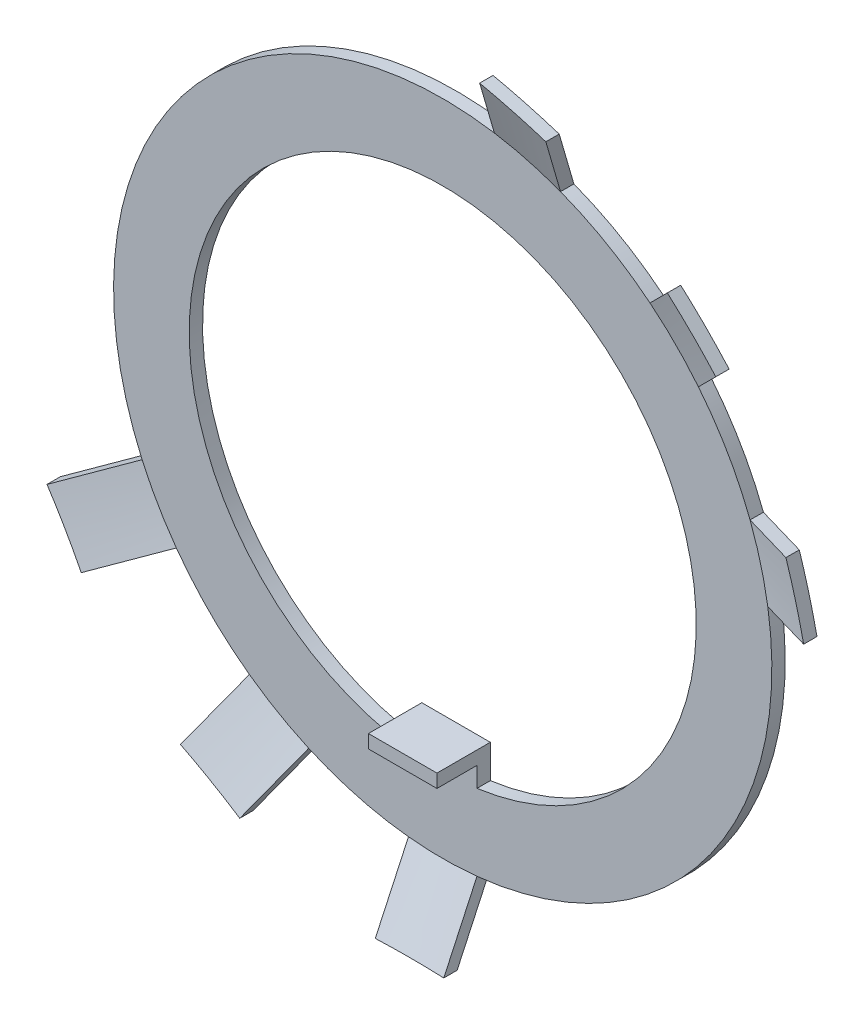
from build123d import *

# Parameters (mm, degrees)
SKETCH3_OUTSIDE_W   = 117.478
SKETCH3_OUTSIDE_H   = 117.478
CUT_EXTRUDE2_DEPTH  = 5.230463
SKETCH4_W           = 7.7
SKETCH4_H           = 1.5
BOSS_EXTRUDE1_DEPTH = 6


with BuildPart() as part:
    # Sketch2 → Boss-Revolve (revolve)
    with BuildSketch(Plane(origin=(0, 0, 0), x_dir=(0, 0, -1), z_dir=(1, 0, 0))):
        Polygon((-3.730461265, 45), (0, 37), (0, 0), (-1.5, 0), (-1.5, 37), (-5.230461265, 45), align=None)
    revolve(axis=Axis((0, 0, 0), (0, 0, 1)))

    # Sketch3 outside → Cut-Extrude2 (cut)
    # profile 1 of 2: a face of its own
    with BuildSketch(Plane.XY):
        Rectangle(SKETCH3_OUTSIDE_W, SKETCH3_OUTSIDE_H)
        with BuildLine():
            Line((-3.85, -36.799150805), (-3.85, -44.835003067))
            Line((-3.85, -44.835003067), (3.85, -44.835003067))
            Line((3.85, -44.835003067), (3.85, -36.799150805))
            ThreePointArc((3.85, -36.799150805), (29.354073591, -22.524172873), (36.541703472, 5.805506641))
            Line((36.541703472, 5.805506641), (44.303740708, 7.88533825))
            Line((44.303740708, 7.88533825), (42.31083406, 15.322967112))
            Line((42.31083406, 15.322967112), (34.548796825, 13.243135503))
            ThreePointArc((34.548796825, 13.243135503), (32.04293994, 18.5), (28.743290184, 23.298567969))
            Line((28.743290184, 23.298567969), (34.425495811, 28.980773595))
            Line((34.425495811, 28.980773595), (28.980773595, 34.425495811))
            Line((28.980773595, 34.425495811), (23.298567969, 28.743290184))
            ThreePointArc((23.298567969, 28.743290184), (18.5, 32.04293994), (13.243135503, 34.548796825))
            Line((13.243135503, 34.548796825), (15.322967112, 42.31083406))
            Line((15.322967112, 42.31083406), (7.88533825, 44.303740708))
            Line((7.88533825, 44.303740708), (5.805506641, 36.541703472))
            ThreePointArc((5.805506641, 36.541703472), (-29.354073591, 22.524172873), (-33.793999435, -15.065377598))
            Line((-33.793999435, -15.065377598), (-40.753251635, -19.083303729))
            Line((-40.753251635, -19.083303729), (-36.903251635, -25.751699338))
            Line((-36.903251635, -25.751699338), (-29.943999435, -21.733773207))
            ThreePointArc((-29.943999435, -21.733773207), (-26.162950904, -26.162950904), (-21.733773207, -29.943999435))
            Line((-21.733773207, -29.943999435), (-25.751699338, -36.903251635))
            Line((-25.751699338, -36.903251635), (-19.083303729, -40.753251635))
            Line((-19.083303729, -40.753251635), (-15.065377598, -33.793999435))
            ThreePointArc((-15.065377598, -33.793999435), (-9.576304669, -35.739255573), (-3.85, -36.799150805))
        make_face(mode=Mode.SUBTRACT)
    # profile 2 of 2: a face of its own
    with BuildSketch(Plane.XY):
        with BuildLine():
            Line((3.85, -28.238758825), (3.85, -24.5))
            Line((3.85, -24.5), (-3.85, -24.5))
            Line((-3.85, -24.5), (-3.85, -28.238758825))
            ThreePointArc((-3.85, -28.238758825), (0, 28.5), (3.85, -28.238758825))
        make_face()
    extrude(amount=CUT_EXTRUDE2_DEPTH, mode=Mode.SUBTRACT)

    # Sketch4 → Boss-Extrude1 (add)
    with BuildSketch(Plane.XY):
        with Locations((0, -25.25)):
            Rectangle(SKETCH4_W, SKETCH4_H)
    extrude(amount=BOSS_EXTRUDE1_DEPTH)


solid = part.part
